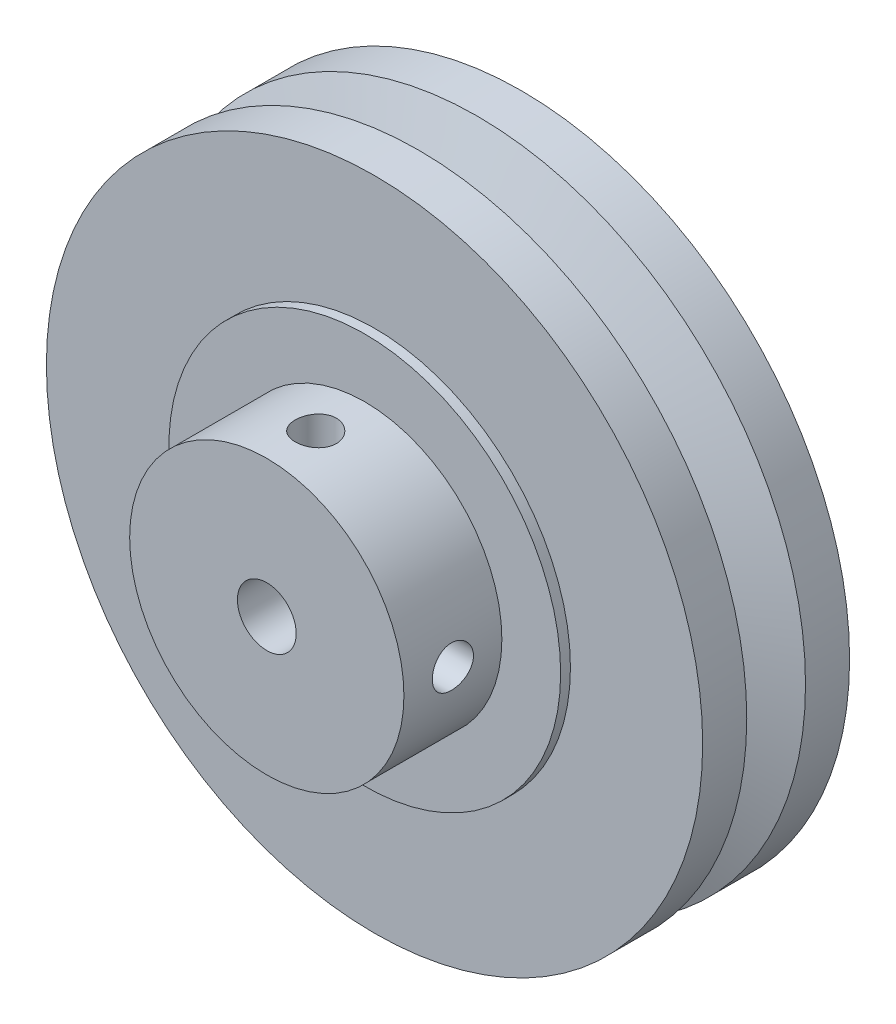
SolidWorks part; units mm, degrees
material "PC"
ref_plane "Front" through (0, 0, 0) normal (0, 0, 1) x (1, 0, 0)
ref_plane "Top" through (0, 0, 0) normal (0, 1, 0) x (1, 0, 0)
ref_plane "Right" through (0, 0, 0) normal (1, 0, 0) x (0, 0, -1)
sketch "Sketch1" plane through (0, 0, 0) normal (0, 0, 1) x (1, 0, 0)
  circle A0 centre (0, 0) radius 33.5
  dimension "D1" = 67
extrude "Boss-Extrude1" add sketch "Sketch1" along normal blind 15
sketch "Sketch2" plane through (0, 0, 15) normal (0, 0, 1) x (1, 0, 0)
  circle A0 centre (0, 0) radius 20
  dimension "D1" = 40
sketch "Sketch3" plane through (0, 0, 0) normal (0, 0, -1) x (-1, 0, 0)
  circle A2 centre (0, 0) radius 20
  circle A3 centre (0, 0) radius 20
  dimension "D1" = 0
sketch "Sketch4" plane through (0, 0, 15) normal (0, 0, 1) x (1, 0, 0)
  circle A0 centre (0, 0) radius 14
  dimension "D1" = 28
extrude "Boss-Extrude2" add sketch "Sketch4" along normal blind 11
extrude "Boss-Extrude4" add sketch "Sketch3" along normal blind 2
extrude "Boss-Extrude3" add sketch "Sketch2" along normal blind 1
sketch "Sketch5" plane through (0, 0, 26) normal (0, 0, 1) x (1, 0, 0)
  circle A0 centre (0, 0) radius 3
  dimension "D1" = 6
extrude "Cut-Extrude3" cut sketch "Sketch5" against normal through all
sketch "Sketch7" plane through (0, 0, 0) normal (1, 0, 0) x (0, 0, -1)
  line L0 (0, 0) -> (-29.3258, 0) construction
  line L1 (-7.5, 33.5) -> (-7.5, 26.85) construction
  line L2 (0, 33.5) -> (-15, 33.5) construction
  line L3 (-8, 26.85) -> (-7, 26.85)
  line L4 (-7, 26.85) -> (-4.5, 33.5)
  line L5 (-4.5, 33.5) -> (-10.5, 33.5)
  line L6 (-8, 26.85) -> (-10.5, 33.5)
  dimension "D1" = 53.7
  dimension "D2" = 1
  dimension "D3" = 6
revolve "Cut-Revolve1" cut sketch "Sketch7" angle 360 about L0
ref_plane "Plane1" through (0, 0, 21) normal (0, 0, 1) x (1, 0, 0)
sketch "Sketch10" plane through (0, 0, 21) normal (0, 0, 1) x (1, 0, 0)
  circle A1 centre (0, 0) radius 14
  circle A2 centre (0, 0) radius 14
  point P0 (0, 14)
  point P1 (14, 0)
  dimension "D1" = 0
hole_wizard "M5 Tapped Hole1" positions "3DSketch2" profile "Sketch12" tap size "M5" standard "GB"
sketch3d "3DSketch2"
  circle A0 centre (0, 0, 21) radius 14 construction
  point P0 (0, 14, 21)
  point P2 (14, 0, 21)
  point P12 (0, 0, 35)
cosmetic thread "Hole thread2" parameters "D1"=10, "D2"=5
cosmetic thread "Hole thread3" parameters "D1"=10, "D2"=5
sketch "Sketch12" plane through (0, 14, 21) normal (1, 0, 0) x (0, 0, 1)
  line L0 (0, 0) -> (0, 14.2618)
  line L1 (0, 14.2618) -> (2.1, 13)
  line L2 (2.1, 13) -> (2.1, 0)
  line L5 (2.1, 0) -> (0, 0)
  line L10 (0, 14.2618) -> (-2.1, 13) construction
  line L11 (0, -6.35) -> (0, 107.95) construction
  dimension "螺纹孔钻头直径" = 4.2
  dimension "螺纹孔钻头深度" = 13
  dimension "导头角度" = 118
